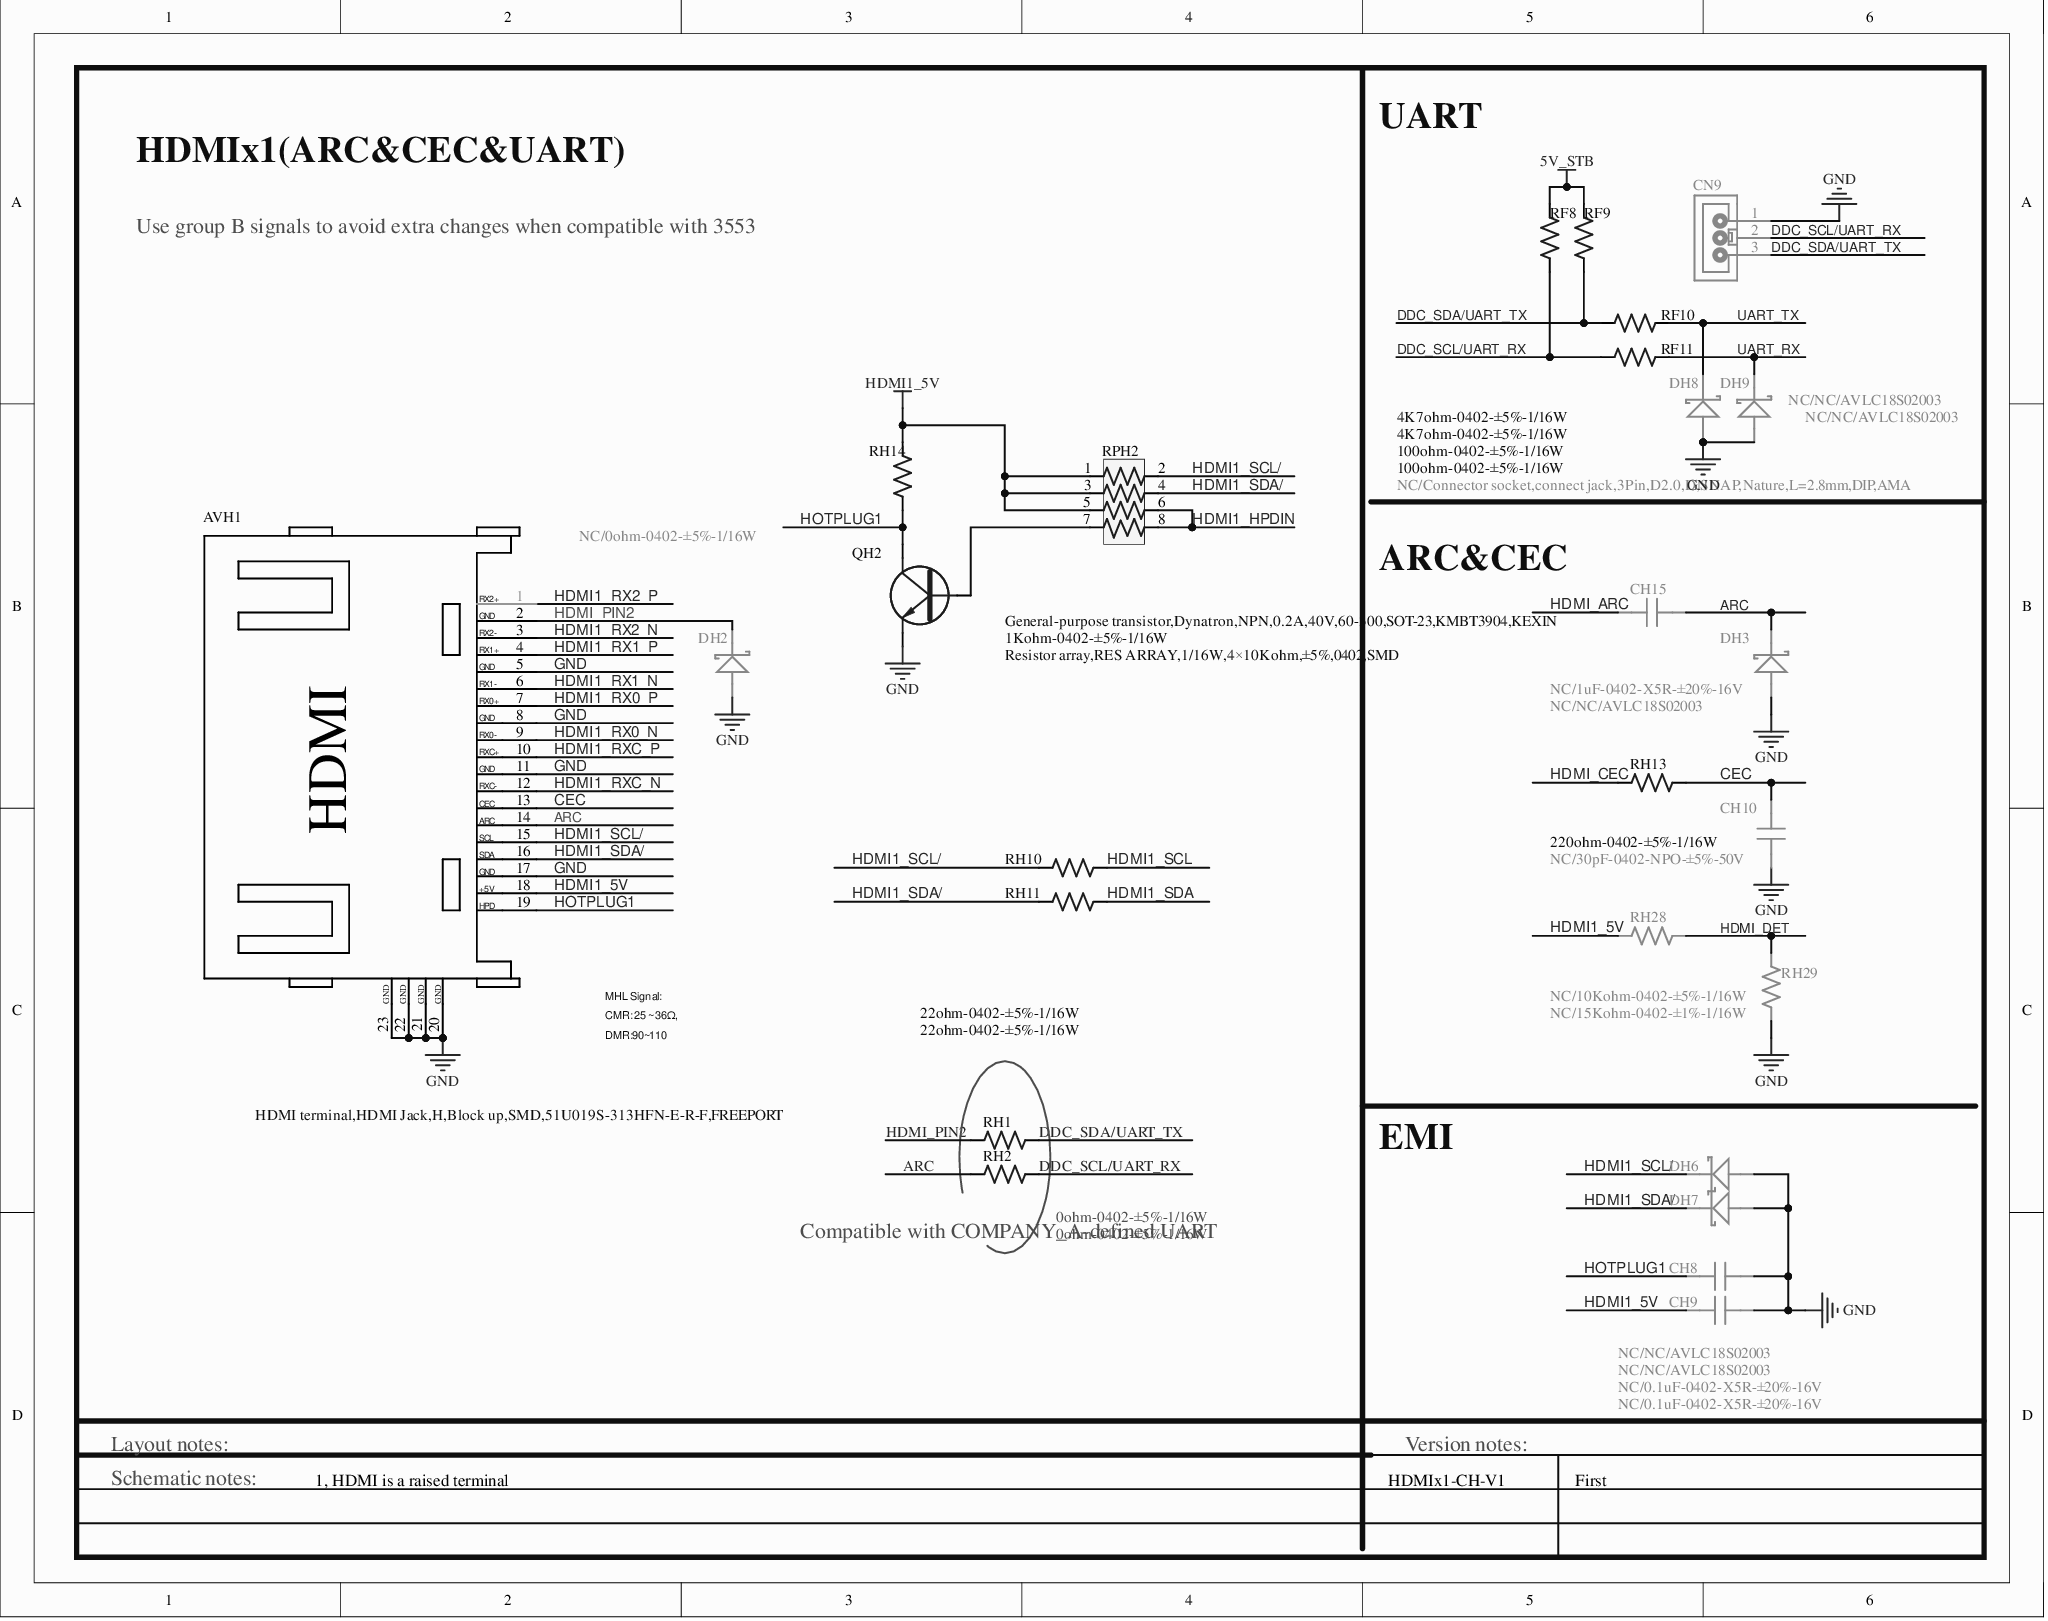
[diagram p0: MISC84438-11.SchDoc]
# Altium project MISC84438-18.PrjPCB (part 6 of 8)

## Sheet MISC84438-11.SchDoc
size 304 x 241 mm

### Parts
AVH1  HDMI terminal,HDMI Jack,H,Block up,SMD,51U019S-313HFN-E-R-F,FREEPORT  [HDMI-HS-11]
CH8  NC/0.1uF-0402-X5R-±20%-16V  [C0402]
CH9  NC/0.1uF-0402-X5R-±20%-16V  [C0402]
CH10  NC/30pF-0402-NPO-±5%-50V  [C0402]
CH15  NC/1uF-0402-X5R-±20%-16V  [C0402]
CN9  NC/Connector socket,connect jack,3Pin,D2.0,D,SNAP,Nature,L=2.8mm,DIP,AMA  [SIP3/2.0D-3]
DH2  NC/0ohm-0402-±5%-1/16W  [DIODE-S0402]
DH3  NC/NC/AVLC18S02003  [DIODE-S0402]
DH6  NC/NC/AVLC18S02003  [DIODE-S0402]
DH7  NC/NC/AVLC18S02003  [DIODE-S0402]
DH8  NC/NC/AVLC18S02003  [DIODE-S0402]
DH9  NC/NC/AVLC18S02003  [DIODE-S0402]
QH2  General-purpose transistor,Dynatron,NPN,0.2A,40V,60-300,SOT-23,KMBT3904,KEXIN  [SOT-23]
RF8  4K7ohm-0402-±5%-1/16W  [R0402]
RF9  4K7ohm-0402-±5%-1/16W  [R0402]
RF10  100ohm-0402-±5%-1/16W  [R0402]
RF11  100ohm-0402-±5%-1/16W  [R0402]
RH1  0ohm-0402-±5%-1/16W  [R0402]
RH2  0ohm-0402-±5%-1/16W  [R0402]
RH10  22ohm-0402-±5%-1/16W  [R0402]
RH11  22ohm-0402-±5%-1/16W  [R0402]
RH13  220ohm-0402-±5%-1/16W  [R0402]
RH14  1Kohm-0402-±5%-1/16W  [R0402]
RH28  NC/10Kohm-0402-±5%-1/16W  [R0402]
RH29  NC/15Kohm-0402-±1%-1/16W  [R0402]
RPH2  Resistor array,RES ARRAY,1/16W,4×10Kohm,±5%,0402,SMD  [RA0402]

### Nets
5V_STB: RF8.2 RF9.2
GND: AVH1.5 AVH1.8 AVH1.11 AVH1.17 AVH1.20 AVH1.21 AVH1.22 AVH1.23 CH8.1 CH9.1 CH10.1 CN9.1 DH2.A DH3.A DH6.A DH7.A DH8.A DH9.A QH2.E RH29.2
HDMI1_5V: AVH1.18 CH9.2 RH14.2 RH28.2 RPH2.1 RPH2.3 RPH2.5
ARC: AVH1.14 CH15.1 DH3.K RH2.1
CEC: AVH1.13 CH10.2 RH13.1
DDC_SCL/UART_RX: CN9.2 RF8.1 RF11.1 RH2.2
DDC_SDA/UART_TX: CN9.3 RF9.1 RF10.1 RH1.2
HDMI1_HPDIN: RPH2.6 RPH2.8
HDMI1_RX0_N: AVH1.9
HDMI1_RX0_P: AVH1.7
HDMI1_RX1_N: AVH1.6
HDMI1_RX1_P: AVH1.4
HDMI1_RX2_N: AVH1.3
HDMI1_RX2_P: AVH1.1
HDMI1_RXC_N: AVH1.12
HDMI1_RXC_P: AVH1.10
HDMI1_SCL: RH10.1
HDMI1_SCL/: AVH1.15 DH6.K RH10.2 RPH2.2
HDMI1_SDA: RH11.1
HDMI1_SDA/: AVH1.16 DH7.K RH11.2 RPH2.4
HDMI_ARC: CH15.2
HDMI_CEC: RH13.2
HDMI_DET: RH28.1 RH29.1
HDMI_PIN2: AVH1.2 DH2.K RH1.1
HOTPLUG1: AVH1.19 CH8.2 QH2.C RH14.1
UART_RX: DH9.K RF11.2
UART_TX: DH8.K RF10.2
NetQH2_B: QH2.B RPH2.7

### Notes on the sheet
- HDMIx1(ARC&CEC&UART)
- UART
- Use group B signals to avoid extra changes when compatible with 3553
- ARC&CEC
- MHL Signal:
- CMR: 25 ~36Ω,
- DMR:90~110
- EMI
- (near RH2) Compatible with COMPANY_A-defined UART
- Layout notes:
- Schematic notes:
- 1, HDMI is a raised terminal
- HDMIx1-CH-V1
- Version notes:
- First

### Library data of the parts
AVH1 = XXX.XXX.0001809-D: HDMI terminal,HDMI Jack,H,Block up,SMD,51U019S-313HFN-E-R-F,FREEPORT-D
CH8 CH9 = 0.1uF-0402-Y5V-+80%-20%-16V-D
CH10 = 33pF-0402-NPO-±5%-50V-D
CH15 = 1uF-0402-X5R-±20%-16V-D
CN9 = 3PIN-2.0-D-H-G-带扣-DHMI
DH2 DH3 DH6-DH9 = AVLC18S02003-D
QH2 = MMBT3904(f≥350MHz)-D-NPN: Q-NPN-#-#-#
RF8 RF9 = 4K7ohm-0402-±5%-1/16W-D
RF10 RF11 = 100ohm-0402-±5%-1/16W-D
RH1 RH2 = 0ohm-0402-±5%-1/16W-D
RH10 RH11 = 10Kohm-0402-±5%-1/16W-D
RH13 RH28 RH29 = 220ohm-0402-±5%-1/16W-D
RH14 = 1Kohm-0402-±5%-1/16W-D
RPH2 = 4*100ohm-0402-±5%-1/16W-D

## Sheet MISC84438-12.SchDoc
size 266 x 241 mm
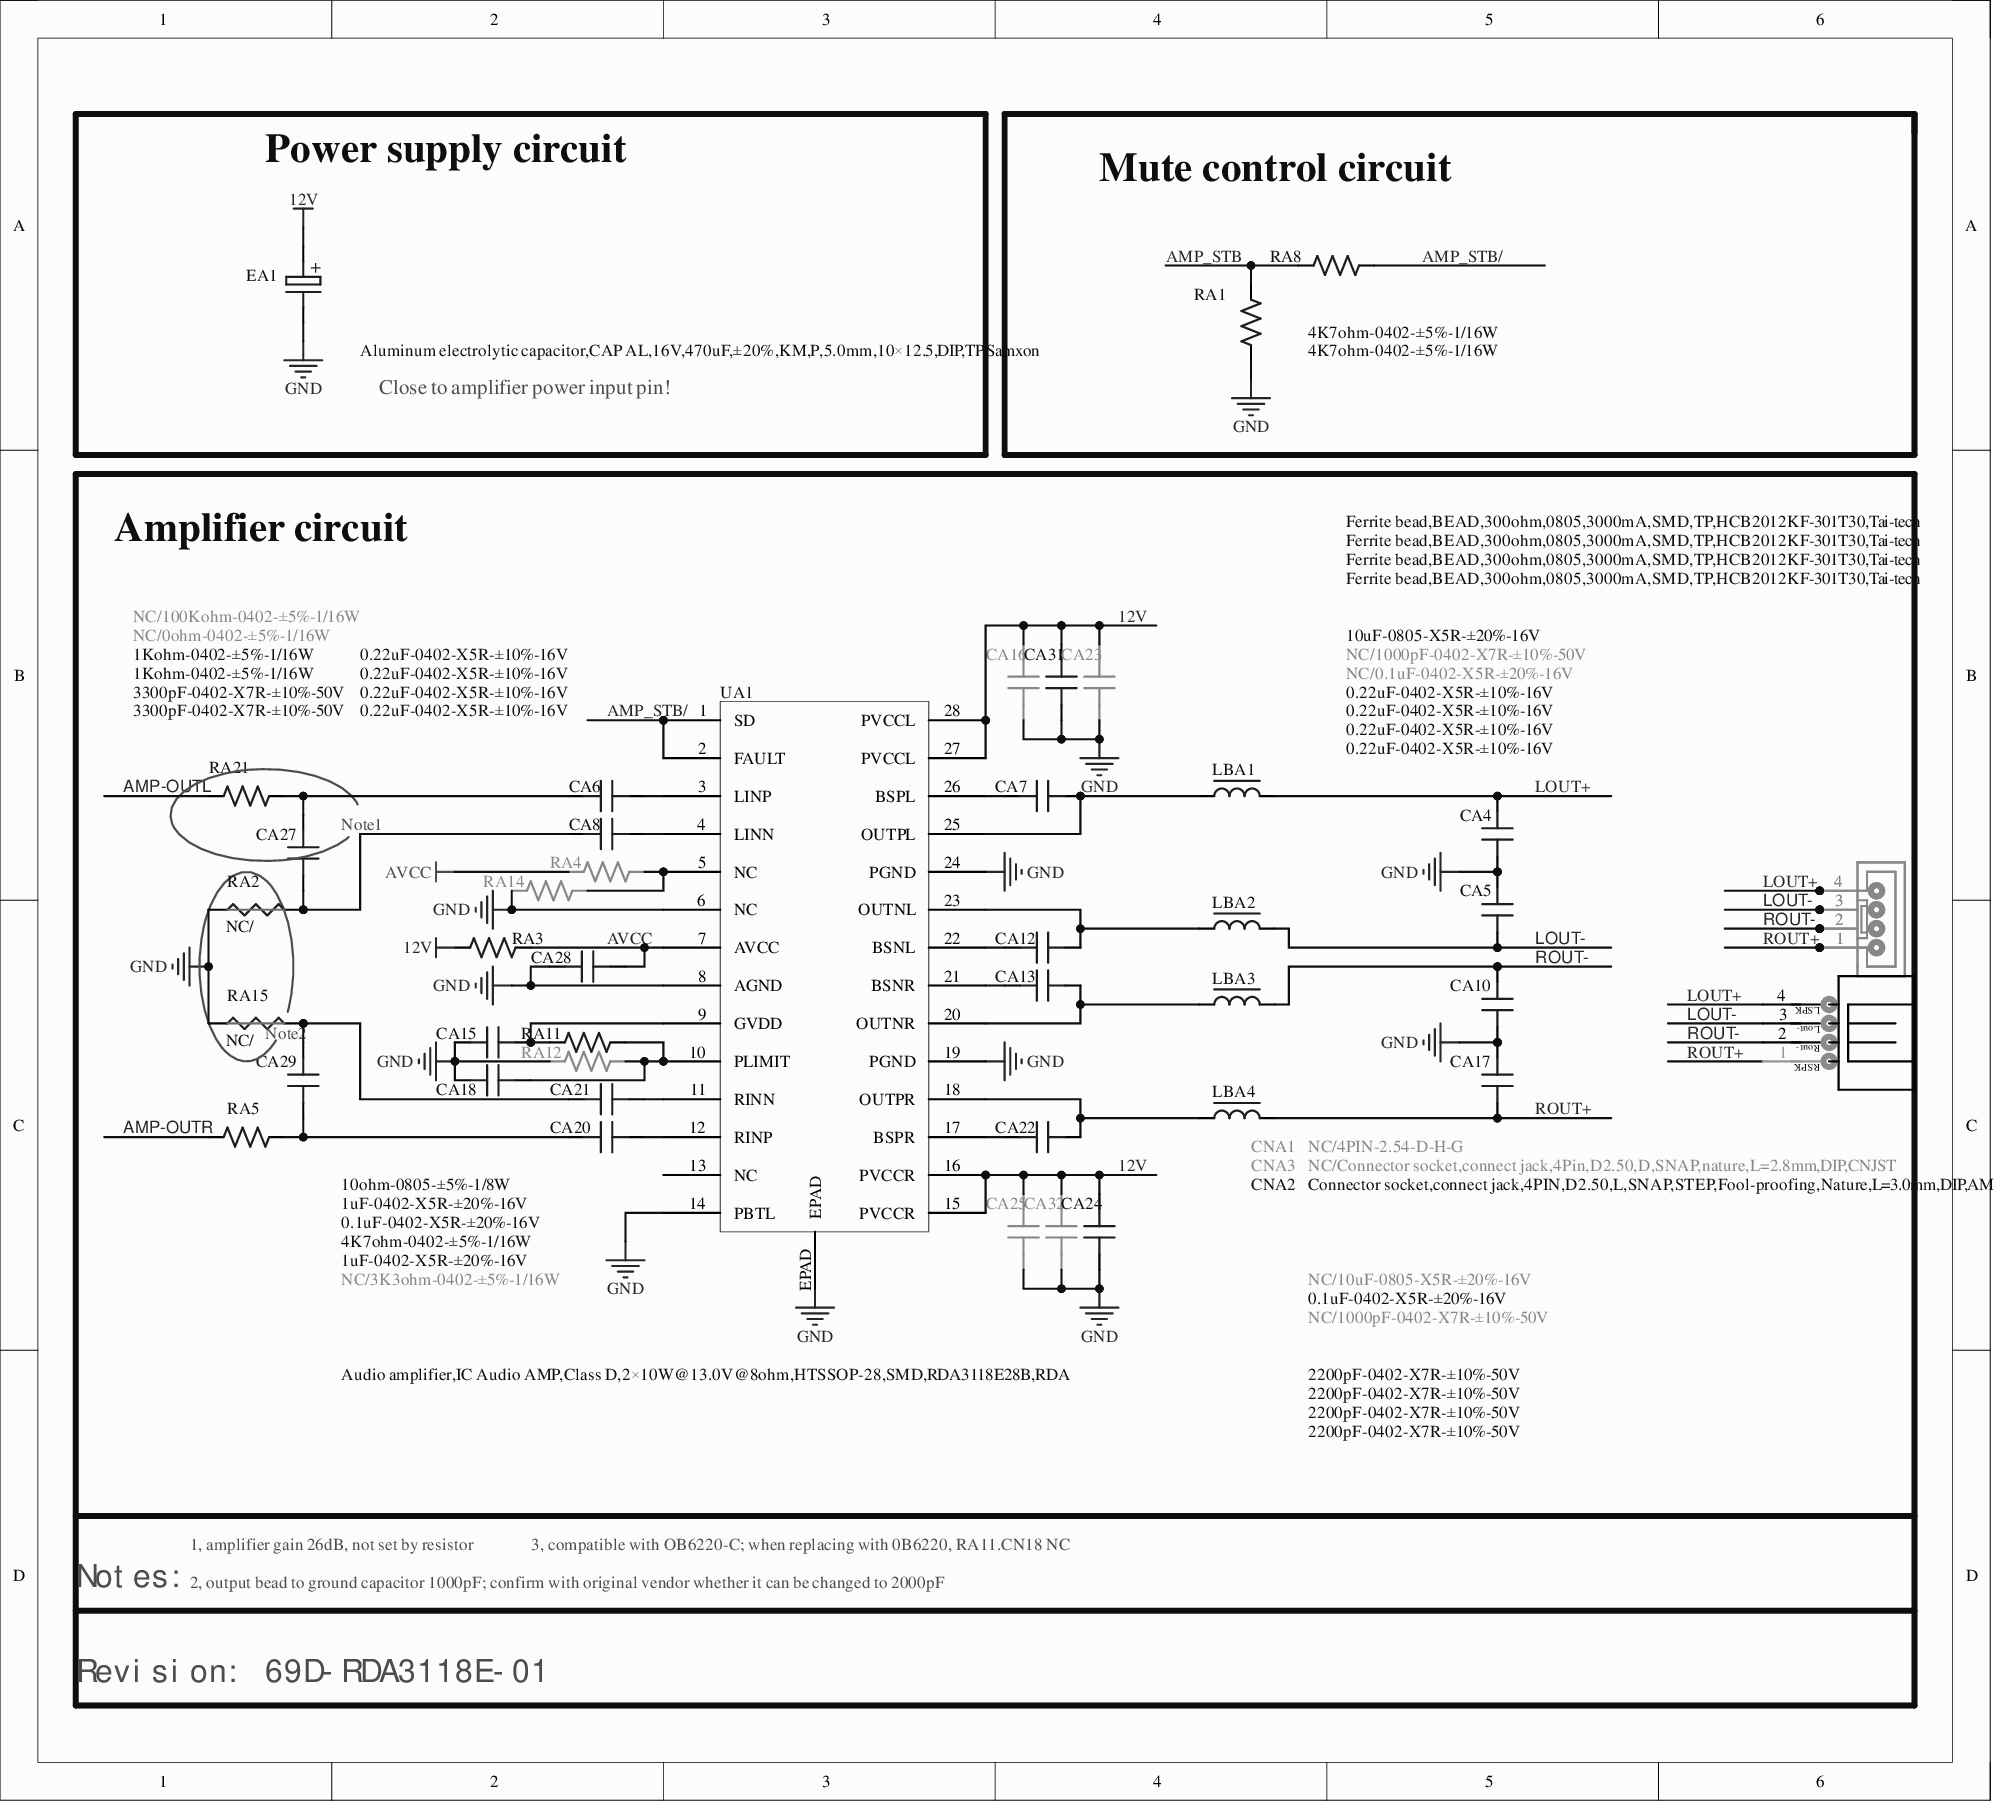
[diagram p1: MISC84438-12.SchDoc]

### Parts
CA4  2200pF-0402-X7R-±10%-50V  [C0402]
CA5  2200pF-0402-X7R-±10%-50V  [C0402]
CA6  0.22uF-0402-X5R-±10%-16V  [C0402]
CA7  0.22uF-0402-X5R-±10%-16V  [C0402]
CA8  0.22uF-0402-X5R-±10%-16V  [C0402]
CA10  2200pF-0402-X7R-±10%-50V  [C0402]
CA12  0.22uF-0402-X5R-±10%-16V  [C0402]
CA13  0.22uF-0402-X5R-±10%-16V  [C0402]
CA15  0.1uF-0402-X5R-±20%-16V  [C0402]
CA16  NC/1000pF-0402-X7R-±10%-50V  [C0402]
CA17  2200pF-0402-X7R-±10%-50V  [C0402]
CA18  1uF-0402-X5R-±20%-16V  [C0402]
CA20  0.22uF-0402-X5R-±10%-16V  [C0402]
CA21  0.22uF-0402-X5R-±10%-16V  [C0402]
CA22  0.22uF-0402-X5R-±10%-16V  [C0402]
CA23  NC/0.1uF-0402-X5R-±20%-16V  [C0402]
CA24  0.1uF-0402-X5R-±20%-16V  [C0402]
CA25  NC/1000pF-0402-X7R-±10%-50V  [C0402]
CA27  3300pF-0402-X7R-±10%-50V  [C0402]
CA28  1uF-0402-X5R-±20%-16V  [C0402]
CA29  3300pF-0402-X7R-±10%-50V  [C0402]
CA31  10uF-0805-X5R-±20%-16V  [C0805]
CA32  NC/10uF-0805-X5R-±20%-16V  [C0805]
CNA1  NC/4PIN-2.54-D-H-G  [SIP4/2.54D-1]
CNA2  Connector socket,connect jack,4PIN,D2.50,L,SNAP,STEP,Fool-proofing,Nature,L=3.0mm,DIP,AMA  [SIP4H/2.54D-2]
CNA3  NC/Connector socket,connect jack,4Pin,D2.50,D,SNAP,nature,L=2.8mm,DIP,CNJST  [SIP4/2.5D-2]
EA1  Aluminum electrolytic capacitor,CAP AL,16V,470uF,±20%,KM,P,5.0mm,10×12.5,DIP,TP,Samxon  [EC(10*12.5)-V-5]
LBA1  Ferrite bead,BEAD,300ohm,0805,3000mA,SMD,TP,HCB2012KF-301T30,Tai-tech  [L0805]
LBA2  Ferrite bead,BEAD,300ohm,0805,3000mA,SMD,TP,HCB2012KF-301T30,Tai-tech  [L0805]
LBA3  Ferrite bead,BEAD,300ohm,0805,3000mA,SMD,TP,HCB2012KF-301T30,Tai-tech  [L0805]
LBA4  Ferrite bead,BEAD,300ohm,0805,3000mA,SMD,TP,HCB2012KF-301T30,Tai-tech  [L0805]
RA1  4K7ohm-0402-±5%-1/16W  [R0402]
RA2  NC/  [GND]
RA3  10ohm-0805-±5%-1/8W  [R0805]
RA4  NC/100Kohm-0402-±5%-1/16W  [R0402]
RA5  1Kohm-0402-±5%-1/16W  [R0402]
RA8  4K7ohm-0402-±5%-1/16W  [R0402]
RA11  4K7ohm-0402-±5%-1/16W  [R0402]
RA12  NC/3K3ohm-0402-±5%-1/16W  [R0402]
RA14  NC/0ohm-0402-±5%-1/16W  [R0402]
RA15  NC/  [GND]
RA21  1Kohm-0402-±5%-1/16W  [R0402]
UA1  Audio amplifier,IC Audio AMP,Class D,2×10W@13.0V@8ohm,HTSSOP-28,SMD,RDA3118E28B,RDA  [SSOP28/0.65-5]

### Blocks framed on the sheet
Power supply circuit: EA1
Amplifier circuit: CA4-CA8 CA10 CA12 CA13 CA15-CA18 CA20-CA25 CA27-CA29 CA31 CA32 CNA1-CNA3 LBA1-LBA4 RA2-RA5 RA11 RA12 RA14 RA15 RA21 UA1

### Nets
12V: CA16.2 CA23.2 CA24.2 CA25.2 CA31.2 CA32.2 EA1.1 RA3.1 UA1.15(PVCCR) UA1.16(PVCCR) UA1.27(PVCCL) UA1.28(PVCCL)
AVCC: CA28.2 RA3.2 RA4.2 UA1.7(AVCC)
GND: CA4.2 CA5.2 CA10.2 CA15.2 CA16.1 CA17.1 CA18.2 CA23.1 CA24.1 CA25.1 CA28.1 CA31.1 CA32.1 EA1.2 RA1.1 RA2.JP_2K RA12.2 RA14.1 RA15.JP_2K UA1.6(NC) UA1.8(AGND) UA1.14(PBTL) UA1.19(PGND) UA1.24(PGND) UA1.EPAD
AMP-OUTL: RA21.1
AMP-OUTR: RA5.1
AMP_STB: RA1.2 RA8.1
AMP_STB/: RA8.2 UA1.1(SD) UA1.2(FAULT)
LOUT+: CA4.1 CNA1.4 CNA2.4 CNA3.4 LBA1.2
LOUT-: CA5.1 CNA1.3 CNA2.3 CNA3.3 LBA2.2
ROUT+: CA17.2 CNA1.1 CNA2.1 CNA3.1 LBA4.2
ROUT-: CA10.1 CNA1.2 CNA2.2 CNA3.2 LBA3.2
NetCA6_1: CA6.1 UA1.3(LINP)
NetCA6_2: CA6.2 CA27.1 RA21.2
NetCA7_1: CA7.1 UA1.26(BSPL)
NetCA7_2: CA7.2 LBA1.1 UA1.25(OUTPL)
NetCA8_1: CA8.1 UA1.4(LINN)
NetCA8_2: CA8.2 CA27.2 RA2.JP_1K
NetCA12_1: CA12.1 UA1.22(BSNL)
NetCA12_2: CA12.2 LBA2.1 UA1.23(OUTNL)
NetCA13_1: CA13.1 UA1.21(BSNR)
NetCA13_2: CA13.2 LBA3.1 UA1.20(OUTNR)
NetCA15_1: CA15.1 RA11.2 UA1.9(GVDD)
NetCA18_1: CA18.1 RA11.1 RA12.1 UA1.10(PLIMIT)
NetCA20_1: CA20.1 UA1.12(RINP)
NetCA20_2: CA20.2 CA29.1 RA5.2
NetCA21_1: CA21.1 UA1.11(RINN)
NetCA21_2: CA21.2 CA29.2 RA15.JP_1K
NetCA22_1: CA22.1 UA1.17(BSPR)
NetCA22_2: CA22.2 LBA4.1 UA1.18(OUTPR)
NetRA4_1: RA4.1 RA14.2 UA1.5(NC)

Not connected (* = marked no-connect by the designer): UA1 13(NC)*

### Notes on the sheet
- Mute control circuit
- Close to amplifier power input pin!
- (near CA27) Note1
- (near RA15) Note2
- 1, amplifier gain 26dB, not set by resistor
- 3, compatible with OB6220-C; when replacing with 0B6220, RA11.CN18 NC
- Notes:
- 2, output bead to ground capacitor 1000pF; confirm with original vendor whether it can be changed to 2000pF
- Revision: 69D-RDA3118E-01

### Library data of the parts
CA4 CA5 CA10 CA16 CA17 CA25 CA27 CA29 = 1000pF-0402-X7R-±10%-50V-D
CA6 CA8 CA20 CA21 = 0.22uF-0402-X5R-±10%-16V-D
CA7 CA12 CA13 CA22 = 0.22uF-0402-Y5V-+80%-20%-16V-D
CA15 CA18 = 1uF-0402-X5R-±20%-16V-D
CA23 CA24 CA28 = 0.1uF-0402-Y5V-+80%-20%-16V-D
CA31 CA32 = 10uF-0603-X5R-±20%-6.3V-D
CNA1 = 4PIN-2.54-D-H-G-DHMI
CNA2 = XXX.XXX.0000738-DLMI-SPEAKER: Connector socket,connect jack,4Pin,D2.50,L,L=2.8mm,DIP,CNJST-DLMI
CNA3 = 4PIN-2.54-D-H-G-带扣-B-DHMI
EA1 = 470uF-25V-±20%-10×12-105℃-YE-编带-F=5.0(Elite)-DHAI: Electrolytic
LBA1-LBA4 = 300ohm-2500mA-0805-D
RA1 RA8 = 100ohm-0402-±5%-1/16W-D
RA2 RA15 = GND: Manufacturer: Panasonic; Part Number: ERJ3GEYJ473V; Right: 20; Bottom: 30; CLASS: Discrete; Comments: Digikey
RA3 = 10ohm-0805-±5%-1/8W-D
RA4 = 47Kohm-0402-±5%-1/16W-D
RA5 RA21 = 180ohm-0402-±5%-1/16W-D
RA11 = 12Kohm-0402-±5%-1/16W-D
RA12 = 9K1ohm-0402-±5%-1/16W-D
RA14 = 0ohm-0402-±5%-1/16W-D
UA1 = 音频功放,IC Audio AMP,Class D,2×9W@13V@8ohm,HTSSOP28,SMD,TPA3136D2,TI-D

## Sheet MISC84438-13.SchDoc
size 457 x 266 mm
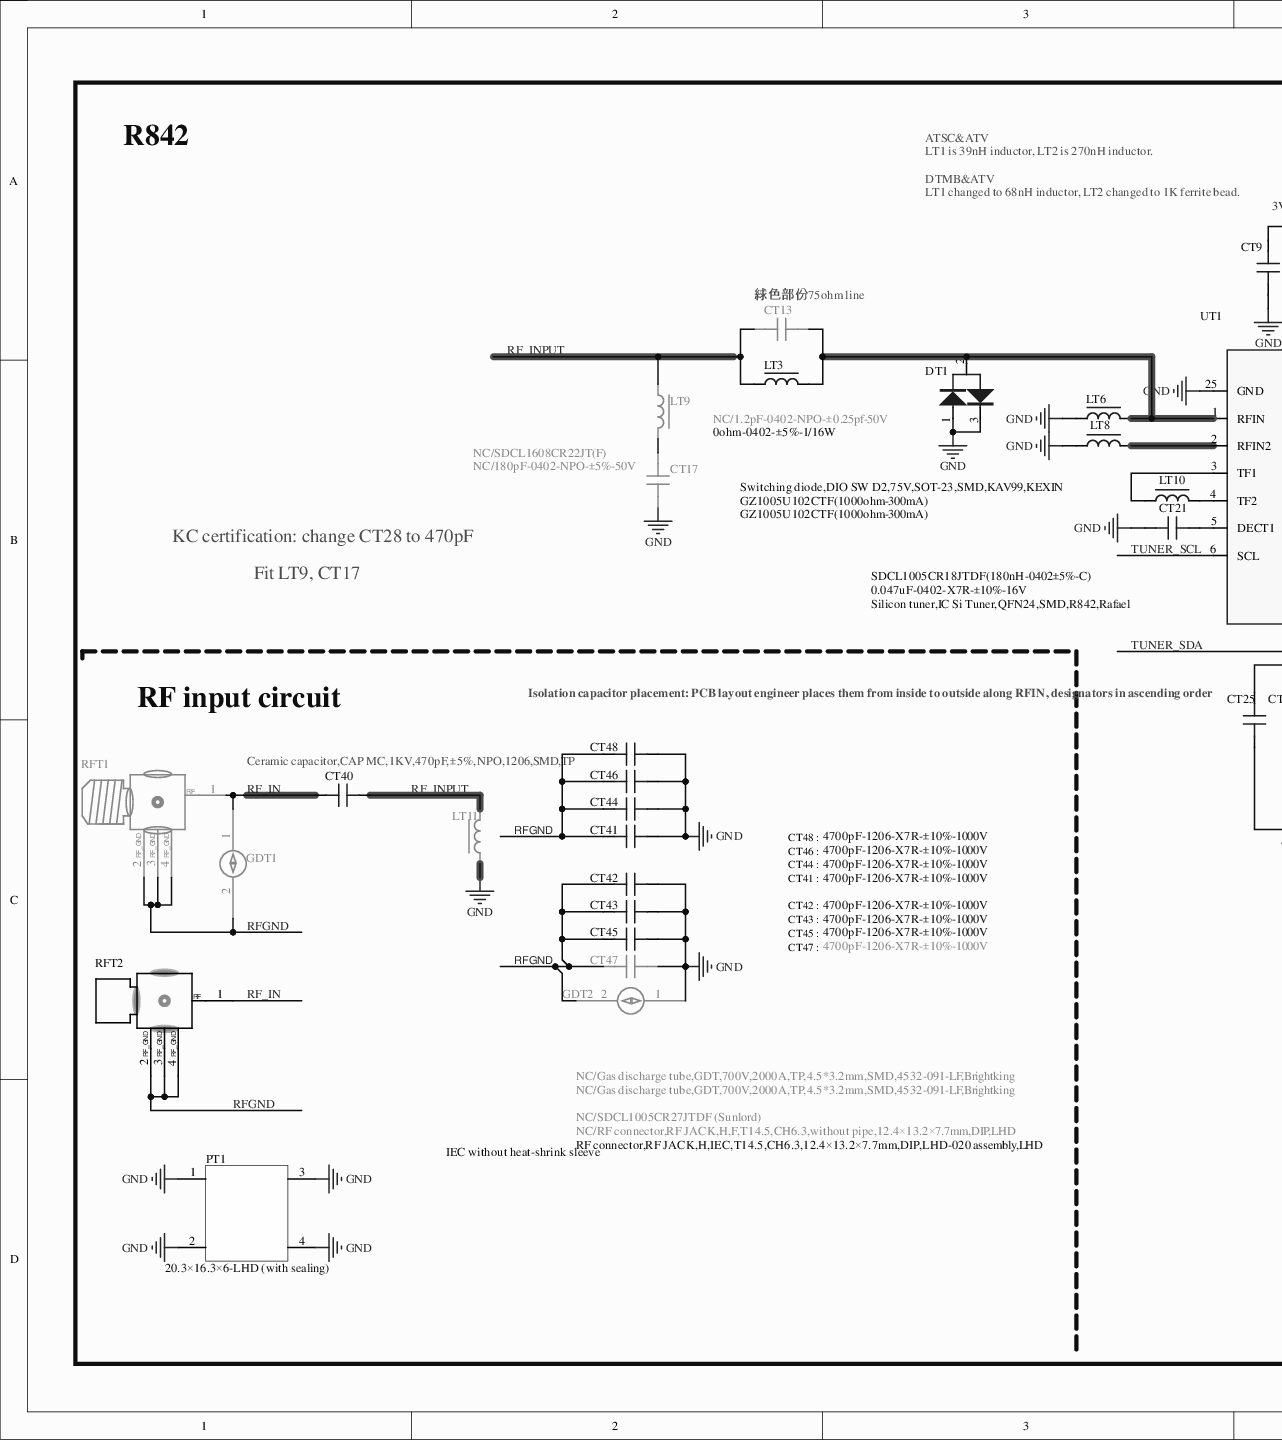
[diagram p2: MISC84438-13.SchDoc, left]
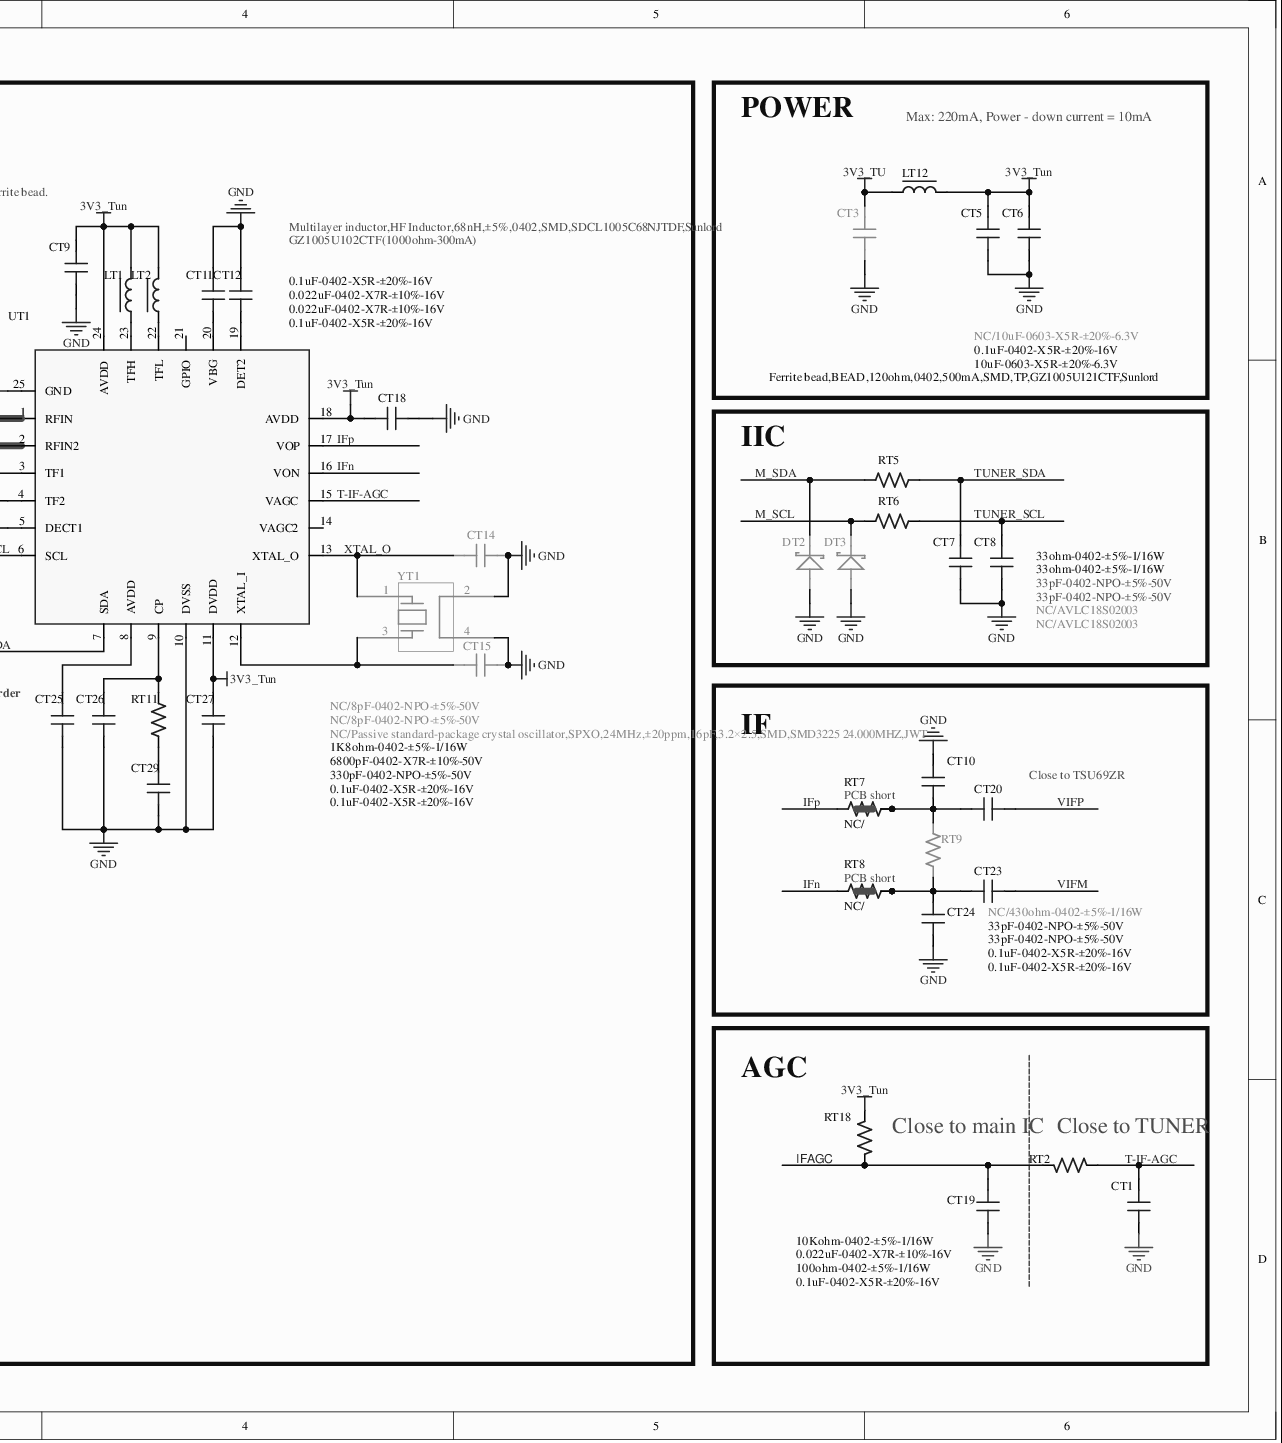
[diagram p3: MISC84438-13.SchDoc, right]

### Parts
CT1  0.1uF-0402-X5R-±20%-16V  [C0402]
CT3  NC/10uF-0603-X5R-±20%-6.3V  [C0603]
CT5  0.1uF-0402-X5R-±20%-16V  [C0402]
CT6  10uF-0603-X5R-±20%-6.3V  [C0603]
CT7  33pF-0402-NPO-±5%-50V  [C0402]
CT8  33pF-0402-NPO-±5%-50V  [C0402]
CT9  0.1uF-0402-X5R-±20%-16V  [C0402]
CT10  33pF-0402-NPO-±5%-50V  [C0402]
CT11  0.022uF-0402-X7R-±10%-16V  [C0402]
CT12  0.022uF-0402-X7R-±10%-16V  [C0402]
CT13  NC/1.2pF-0402-NPO-±0.25pf-50V  [C0402]
CT14  NC/8pF-0402-NPO-±5%-50V  [C0402]
CT15  NC/8pF-0402-NPO-±5%-50V  [C0402]
CT17  NC/180pF-0402-NPO-±5%-50V  [C0402]
CT18  0.1uF-0402-X5R-±20%-16V  [C0402]
CT19  0.022uF-0402-X7R-±10%-16V  [C0402]
CT20  0.1uF-0402-X5R-±20%-16V  [C0402]
CT21  0.047uF-0402-X7R-±10%-16V  [C0402]
CT23  0.1uF-0402-X5R-±20%-16V  [C0402]
CT24  33pF-0402-NPO-±5%-50V  [C0402]
CT25  0.1uF-0402-X5R-±20%-16V  [C0402]
CT26  330pF-0402-NPO-±5%-50V  [C0402]
CT27  0.1uF-0402-X5R-±20%-16V  [C0402]
CT29  6800pF-0402-X7R-±10%-50V  [C0402]
CT40  Ceramic capacitor,CAP MC,1KV,470pF,±5%,NPO,1206,SMD,TP  [C1206]
CT41  4700pF-1206-X7R-±10%-1000V  [C1206]
CT42  4700pF-1206-X7R-±10%-1000V  [C1206]
CT43  4700pF-1206-X7R-±10%-1000V  [C1206]
CT44  4700pF-1206-X7R-±10%-1000V  [C1206]
CT45  4700pF-1206-X7R-±10%-1000V  [C1206]
CT46  4700pF-1206-X7R-±10%-1000V  [C1206]
CT47  4700pF-1206-X7R-±10%-1000V  [C1206]
CT48  4700pF-1206-X7R-±10%-1000V  [C1206]
DT1  Switching diode,DIO SW D2,75V,SOT-23,SMD,KAV99,KEXIN  [SO-23]
DT2  NC/AVLC18S02003  [DIODE-S0402]
DT3  NC/AVLC18S02003  [DIODE-S0402]
GDT1  NC/Gas discharge tube,GDT,700V,2000A,TP,4.5*3.2mm,SMD,4532-091-LF,Brightking  [SMD4532-1]
GDT2  NC/Gas discharge tube,GDT,700V,2000A,TP,4.5*3.2mm,SMD,4532-091-LF,Brightking  [SMD4532-1]
LT1  Multilayer inductor,HF Inductor,68nH,±5%,0402,SMD,SDCL1005C68NJTDF,Sunlord  [L0402]
LT2  GZ1005U102CTF(1000ohm-300mA)  [L0402]
LT3  0ohm-0402-±5%-1/16W  [L0402]
LT6  GZ1005U102CTF(1000ohm-300mA)  [L0402]
LT8  GZ1005U102CTF(1000ohm-300mA)  [L0402]
LT9  NC/SDCL1608CR22JT(F)  [L0603]
LT10  SDCL1005CR18JTDF(180nH-0402±5%-C)  [L0402]
LT11  NC/SDCL1005CR27JTDF (Sunlord)  [L0402]
LT12  Ferrite bead,BEAD,120ohm,0402,500mA,SMD,TP,GZ1005U121CTF,Sunlord  [L0402]
PT1  20.3×16.3×6-LHD (with sealing)  [SHIELD(16*20*6)]
RFT1  NC/RF connector,RF JACK,H,F,T14.5,CH6.3,without pipe,12.4×13.2×7.7mm,DIP,LHD  [T-13.2×12.4×7.7-F14.5]
RFT2  RF connector,RF JACK,H,IEC,T14.5,CH6.3,12.4×13.2×7.7mm,DIP,LHD-020 assembly,LHD  [ANT-IEC14.5-H-4]
RT2  100ohm-0402-±5%-1/16W  [R0402]
RT5  33ohm-0402-±5%-1/16W  [R0402]
RT6  33ohm-0402-±5%-1/16W  [R0402]
RT7  NC/  [R0402SC]
RT8  NC/  [R0402SC]
RT9  NC/430ohm-0402-±5%-1/16W  [R0402]
RT11  1K8ohm-0402-±5%-1/16W  [R0402]
RT18  10Kohm-0402-±5%-1/16W  [R0402]
UT1  Silicon tuner,IC Si Tuner,QFN24,SMD,R842,Rafael  [QFN24/0.5-3]
YT1  NC/Passive standard-package crystal oscillator,SPXO,24MHz,±20ppm,16pF,3.2×2.5,SMD,SMD3225 24.000MHZ,JWT  [XTAL-S-10]

### Blocks framed on the sheet
POWER: CT3 CT5 CT6 LT12
IIC: CT7 CT8 DT2 DT3 RT5 RT6
IF: CT10 CT20 CT23 CT24 RT7-RT9
AGC: CT1 CT19 RT2 RT18

### Nets
3V3_TU: CT3.1 LT12.1
3V3_Tun: CT5.2 CT6.1 CT9.1 CT18.2 CT27.1 LT1.1 LT2.2 LT12.2 RT18.1 UT1.11(DVDD) UT1.18(AVDD) UT1.24(AVDD)
GND: CT1.1 CT3.2 CT5.1 CT6.2 CT7.1 CT8.1 CT9.2 CT10.2 CT11.1 CT12.2 CT14.1 CT15.1 CT17.2 CT18.1 CT19.1 CT21.2 CT24.1 CT25.2 CT26.1 CT27.2 CT29.1 CT41.1 CT42.1 CT43.1 CT44.1 CT45.1 CT46.1 CT47.1 CT48.1 DT1.1 DT1.3 DT2.A DT3.A GDT2.1 LT6.2 LT8.2 LT11.2 PT1.1 PT1.2 PT1.3 PT1.4 UT1.10(DVSS) UT1.25(GND) YT1.2 YT1.4
IFAGC: CT19.2 RT2.2 RT18.2
IFn: RT8.1 UT1.16(VON)
IFp: RT7.1 UT1.17(VOP)
M_SCL: DT3.K RT6.1
M_SDA: DT2.K RT5.1
RF_IN: CT40.1 GDT1.1 RFT1.1 RFT2.1
RF_INPUT: CT13.1 CT40.2 LT3.1 LT9.1 LT11.1
RFGND: CT41.2 CT42.2 CT43.2 CT44.2 CT45.2 CT46.2 CT47.2 CT48.2 GDT1.2 GDT2.2 RFT1.2 RFT1.3 RFT1.4 RFT2.2 RFT2.3 RFT2.4
T-IF-AGC: CT1.2 RT2.1 UT1.15(VAGC)
TUNER_SCL: CT8.2 RT6.2 UT1.6(SCL)
TUNER_SDA: CT7.2 RT5.2 UT1.7(SDA)
VIFM: CT23.2
VIFP: CT20.2
XTAL_O: CT14.2 UT1.13(XTAL_O) YT1.1
NetCT10_1: CT10.1 CT20.1 RT7.2 RT7.3 RT9.1
NetCT11_2: CT11.2 UT1.20(VBG)
NetCT12_1: CT12.1 UT1.19(DET2)
NetCT13_2: CT13.2 DT1.2 LT3.2 LT6.1 UT1.1(RFIN)
NetCT15_2: CT15.2 UT1.12(XTAL_I) YT1.3
NetCT17_1: CT17.1 LT9.2
NetCT21_1: CT21.1 UT1.5(DECT1)
NetCT23_1: CT23.1 CT24.2 RT8.2 RT8.3 RT9.2
NetCT25_1: CT25.1 UT1.8(AVDD)
NetCT26_2: CT26.2 RT11.2 UT1.9(CP)
NetCT29_2: CT29.2 RT11.1
NetLT1_2: LT1.2 UT1.23(TFH)
NetLT2_1: LT2.1 UT1.22(TFL)
NetLT8_1: LT8.1 UT1.2(RFIN2)
NetLT10_1: LT10.1 UT1.4(TF2)
NetLT10_2: LT10.2 UT1.3(TF1)

Not connected (* = marked no-connect by the designer): UT1 14(VAGC2)* 21(GPIO)*

### Notes on the sheet
- R842
- ATSC&ATV
- LT1 is 39nH inductor, LT2 is 270nH inductor.
- Max: 220mA, Power - down current = 10mA
- DTMB&ATV
- (near CT9) LT1 changed to 68nH inductor, LT2 changed to 1K ferrite bead.
- (near CT13) 絿色部份75ohm line
- KC certification: change CT28 to 470pF
- Fit LT9, CT17
- RF input circuit
- Isolation capacitor placement: PCB layout engineer places them from inside to outside along RFIN, designators in ascending order
- (near CT20) Close to TSU69ZR
- CT48 :
- CT41 :
- CT42 :
- CT43 :
- CT44 :
- CT46 :
- CT45 :
- CT47 :
- IEC without heat-shrink sleeve
- Close to main IC
- (near RT2) Close to TUNER

### Library data of the parts
CT1 CT5 CT9 CT11 CT18 CT20 CT21 CT23 CT25 CT27 = 0.1uF-0402-Y5V-+80%-20%-16V-D
CT3 CT6 = 10uF-0603-X5R-±20%-6.3V-D
CT7 CT8 = 33pF-0402-NPO-±5%-50V-D
CT10 CT24 = 56pF-0402-NPO-±5%-50V-D
CT12 CT19 = 0.022uF-0402-X7R-±10%-16V-D
CT13 = 1.8pF-0402-NPO-±0.25pF-50V-D
CT14 CT15 = 8pF-0402-NPO-±5%-50V-D
CT17 = 120pF-0402-NPO-±5%-50V-D
CT26 = 330pF-0402-NPO-±5%-50V-D
CT29 = 6800pF-0402-X7R-±10%-50V-D
CT40 = 4700pF-1206-X7R-±10%-1000V-D
CT41-CT48 = 1000pF-1206-X7R-±20%-2000V-D
DT1 = BAV99-BR-D
DT2 DT3 = AVLC18S02003-D
GDT1 GDT2 = 004.005.0000675: Gas discharge tube,GDT,700V,2000A,TP,4.5*3.2mm,SMD,4532-091-LF,Brightking-D
LT1 = SDCL1005C68NJTDF(68nH-0402±5%-C)-D
LT2 LT6 LT8 = 1Kohm-0402-±25%-D
LT3 = 2.2nH-0402-±0.3nH-1/4-D
LT9 = SDCL1005CR33JTDF-D
LT10 = SDCL1608CR22JT(F)-D
LT11 = SDCL1005CR27JTDF(顺络)-D
LT12 = GZ1005U121CTF(120ohm-500mA)-D
PT1 = 20.3×16.3×6-LHD(带封口)-DMI
RFT1 = RF头,RF JACK,H,F,T14.5,CH6.3,without pipe,12.4×13.2×7.7mm,DIP,LHD-DLMI: T-F-6.3mm-#-#
RFT2 = RF头,RF JACK,H,IEC,T14.5,CH6.3,12.4×13.2×7.7mm,DIP,LHD-020组件,LHD-DLMI: T-IEC-6.3mm-#-#
RT2 RT18 = 10Kohm-0402-±5%-1/16W-D
RT5 RT6 = 33ohm-0402-±5%-1/16W-D
RT7 RT8 = 0ohm-0402-PCB-D
RT9 = 220ohm-0402-±5%-1/16W-D
RT11 = 1K8ohm-0402-±5%-1/16W-D
UT1 = R840-D
YT1 = 004.009.0000056: Passive standard-package crystal oscillator,SPXO,24MHz,±20ppm,16pF,3.2×2.5,SMD,SMD3225 24.000MHZ,JWT-D